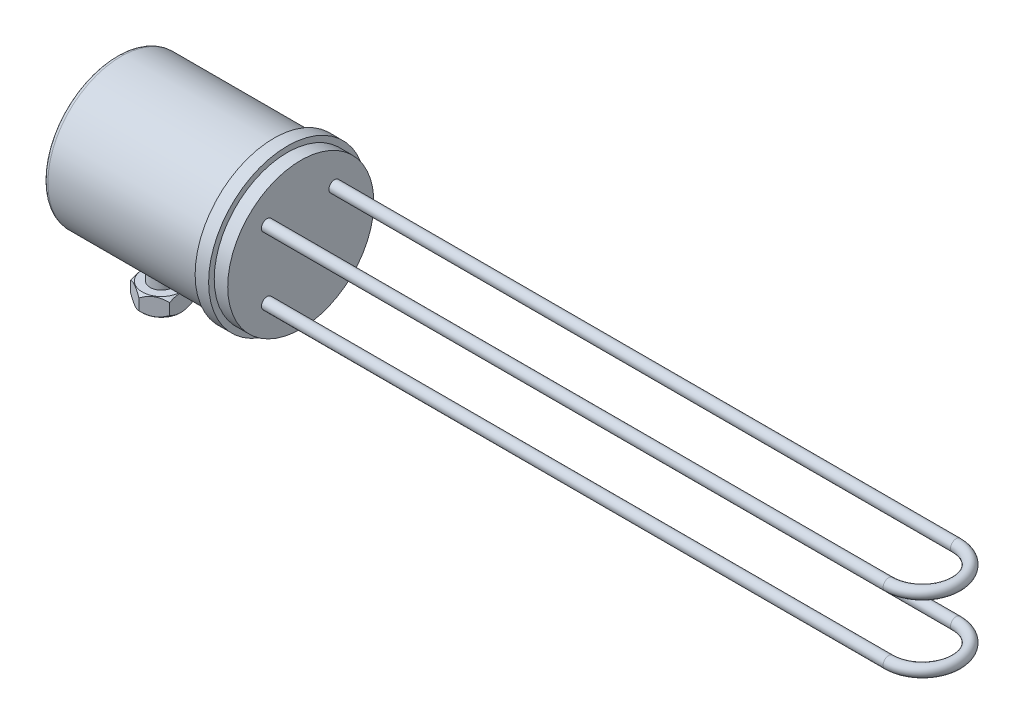
from build123d import *

# Parameters (mm, degrees)
SKETCH1_R           = 2.5
SKETCH3_R           = 32.5
BOSS_EXTRUDE1_DEPTH = 6
SKETCH5_R           = 4.5
CUT_EXTRUDE1_DEPTH  = 6
CIRPATTERN1_COUNT   = 6
SKETCH6_R           = 5
BOSS_EXTRUDE2_DEPTH = 45
SKETCH7_R           = 10
BOSS_EXTRUDE3_DEPTH = 8
CHAMFER1_SIZE       = 1.5
CUT_EXTRUDE2_START  = -8
CUT_EXTRUDE2_DEPTH  = 8
FILLET1_R           = 2
SKETCH9_R           = 57.5
SKETCH9_R_2         = 35
CUT_EXTRUDE3_DEPTH  = 323.720467373


with BuildPart() as part:
    # Sweep1: sweep along a path in Sketch2
    with BuildLine(Plane(origin=(0, 0, 0), x_dir=(1, 0, 0), z_dir=(0, 1, 0))) as sweep1_path:
        Line((0, 0), (282.5, 0))
        ThreePointArc((282.5, 0), (297.5, 15), (282.5, 30))
        Line((282.5, 30), (0, 30))
    # Sketch1 → Sweep1 (sweep)
    with BuildSketch(Plane(origin=(0, 0, 0), x_dir=(0, 0, -1), z_dir=(1, 0, 0))):
        Circle(SKETCH1_R)
    sweep1 = sweep(path=sweep1_path.line)

    # Sketch3 → Boss-Extrude1 (add)
    with BuildSketch(Plane.ZY):
        with Locations((-15, -15)):
            Circle(SKETCH3_R)
    extrude(amount=-BOSS_EXTRUDE1_DEPTH)

    # Mirror3: Sweep1 across plane
    add(sweep1.mirror(Plane.ZX.offset(-15)))

    # Sketch4 → Revolve1 (revolve)
    with BuildSketch(Plane(origin=(0, -15, 0), x_dir=(-1, 0, 0), z_dir=(0, 1, 0))):
        Polygon((0, -15), (0, 42.5), (6, 42.5), (6, 17.5), (76, 17.5), (76, -5), (78, -5), (78, -15), align=None)
    revolve(axis=Axis((-78, -15, -15), (1, 0, 0)))

    # Sketch5 → Cut-Extrude1 (cut)
    with BuildSketch(Plane.ZY.offset(6)):
        with Locations((-15, 32)):
            Circle(SKETCH5_R)
    cut_extrude1 = extrude(amount=-CUT_EXTRUDE1_DEPTH, mode=Mode.SUBTRACT)

    # CirPattern1: Cut-Extrude1 ×6 about axis
    cirpattern1_axis = Axis((0, -15, -15), (1, 0, 0))
    for i in range(1, CIRPATTERN1_COUNT):
        add(cut_extrude1.rotate(cirpattern1_axis, i * 360 / CIRPATTERN1_COUNT), mode=Mode.SUBTRACT)

    # Sketch6 → Boss-Extrude2 (add)
    with BuildSketch(Plane(origin=(0, -15, 0), x_dir=(-1, 0, 0), z_dir=(0, 1, 0))):
        with Locations(Location((56, -15, 0), (0, 0, 90))):
            Circle(SKETCH6_R)
    extrude(amount=-BOSS_EXTRUDE2_DEPTH)

    # Sketch7 → Boss-Extrude3 (add)
    with BuildSketch(Plane.XZ.offset(60)):
        with Locations(Location((-56, -15, 0), (0, 0, 270))):
            Circle(SKETCH7_R)
    extrude(amount=BOSS_EXTRUDE3_DEPTH)

    # Chamfer1
    chamfer1_edges = [part.edges().sort_by_distance(p)[0] for p in [
        (-56, -60, -5),
        (-56, -68, -5),
    ]]
    chamfer(chamfer1_edges, length=CHAMFER1_SIZE)

    # Sketch8 → Cut-Extrude2 (cut)
    with BuildSketch(Plane.XZ.offset(68).offset(CUT_EXTRUDE2_START)):
        with BuildLine():
            Line((-64.660254038, -20), (-64.660254038, -10))
            ThreePointArc((-64.660254038, -10), (-66, -15), (-64.660254038, -20))
        make_face()
        with BuildLine():
            Line((-64.660254038, -10), (-56, -5))
            ThreePointArc((-56, -5), (-61, -6.339745962), (-64.660254038, -10))
        make_face()
        with BuildLine():
            ThreePointArc((-47.339745962, -10), (-51, -6.339745962), (-56, -5))
            Line((-56, -5), (-47.339745962, -10))
        make_face()
        with BuildLine():
            ThreePointArc((-46, -15), (-46.340741737, -12.411809549), (-47.339745962, -10))
            Line((-47.339745962, -10), (-47.339745962, -20))
            ThreePointArc((-47.339745962, -20), (-46.340741737, -17.588190451), (-46, -15))
        make_face()
        with BuildLine():
            ThreePointArc((-56, -25), (-51, -23.660254038), (-47.339745962, -20))
            Line((-47.339745962, -20), (-56, -25))
        make_face()
        with BuildLine():
            Line((-56, -25), (-64.660254038, -20))
            ThreePointArc((-64.660254038, -20), (-61, -23.660254038), (-56, -25))
        make_face()
    extrude(amount=CUT_EXTRUDE2_DEPTH, mode=Mode.SUBTRACT)

    # Fillet1
    fillet1_edges = [part.edges().sort_by_distance(p)[0] for p in [
        (-76, -15, -47.5),
    ]]
    fillet(fillet1_edges, radius=FILLET1_R)

    # Sketch9 → Cut-Extrude3 (cut, through all)
    with BuildSketch(Plane.ZY.offset(6)):
        with Locations((-15, -15)):
            Circle(SKETCH9_R)
        with Locations((-15, -15)):
            Circle(SKETCH9_R_2, mode=Mode.SUBTRACT)
    extrude(amount=-CUT_EXTRUDE3_DEPTH, mode=Mode.SUBTRACT)


solid = part.part
